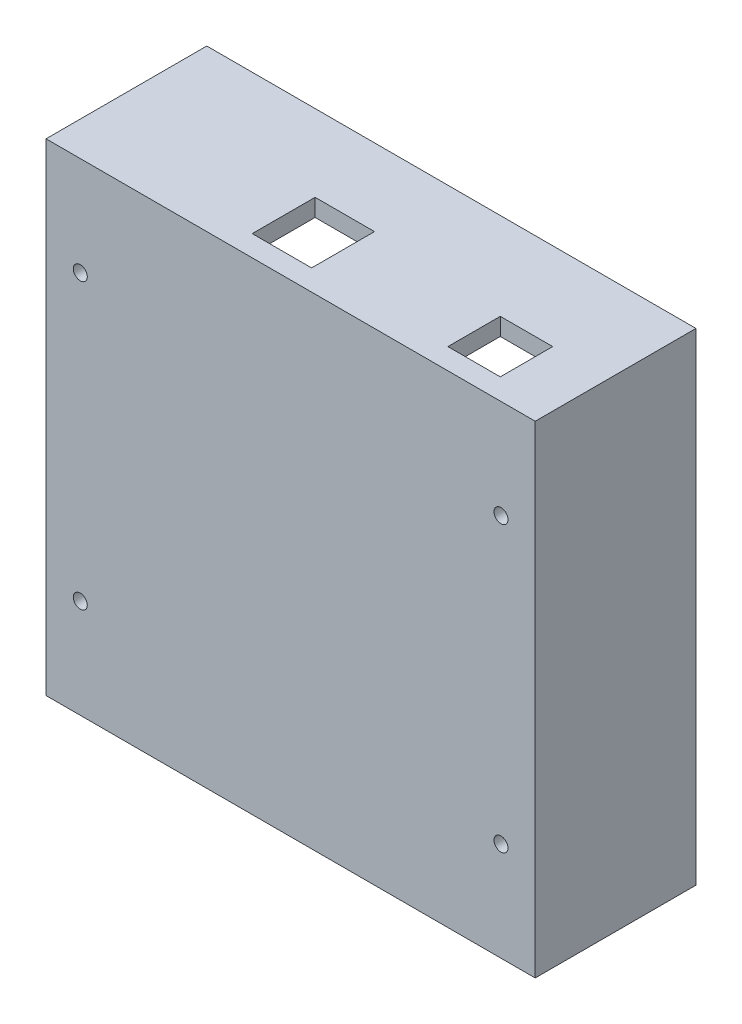
SolidWorks part; units mm, degrees
ref_plane "Front Plane" through (0, 0, 0) normal (0, 0, 1) x (1, 0, 0)
ref_plane "Top Plane" through (0, 0, 0) normal (0, 1, 0) x (1, 0, 0)
ref_plane "Right Plane" through (0, 0, 0) normal (1, 0, 0) x (0, 0, -1)
other "Configuration Table"
sketch "Sketch1" plane through (0, 0, 0) normal (0, 0, 1) x (1, 0, 0)
  line L1 (-47.3118, 118.1115) -> (92.6882, 118.1115)
  line L2 (-47.3118, 118.1115) -> (-47.3118, -19.8885)
  line L3 (-47.3118, -19.8885) -> (92.6882, -19.8885)
  line L4 (92.6882, 118.1115) -> (92.6882, -19.8885)
extrude "Boss-Extrude1" add sketch "Sketch1" along normal blind 46
shell "Shell1" thickness 5
sketch "Sketch8" plane through (0, 118.1115, 0) normal (0, 1, 0) x (1, 0, 0)
  line L0 (-47.3118, -46) -> (-39.3118, -46)
  line L1 (92.6882, -46) -> (-47.3118, -46) construction
sketch "Sketch9" plane through (0, 118.1115, 0) normal (0, 1, 0) x (1, 0, 0)
  line L0 (-39.3118, -46) -> (-39.3118, -40)
  line L6 (-39.3118, -40) -> (-29.3118, -40)
  line L7 (-39.3118, -40) -> (-39.3118, -30)
  line L8 (-39.3118, -30) -> (-29.3118, -30)
  line L9 (-29.3118, -40) -> (-29.3118, -30)
extrude "Cut-Extrude2" cut sketch "Sketch9" against normal blind 5 contours L6 L9 L8 L7
sketch "Sketch10" plane through (0, 118.1115, 0) normal (0, 1, 0) x (1, 0, 0)
  line L0 (-29.3118, -40) -> (-27.3118, -40)
  line L2 (-27.3118, -40) -> (3.6882, -40)
  line L3 (-27.3118, -40) -> (-27.3118, -18)
  line L4 (-27.3118, -18) -> (3.6882, -18)
  line L5 (3.6882, -40) -> (3.6882, -18)
extrude "Cut-Extrude3" cut sketch "Sketch10" against normal blind 5 contours L2 L5 L4 L3
sketch "Sketch11" plane through (0, 118.1115, 0) normal (0, 1, 0) x (1, 0, 0)
  line L0 (3.6882, -40) -> (5.6882, -40)
  line L2 (5.6882, -40) -> (22.6882, -40)
  line L3 (5.6882, -40) -> (5.6882, -22)
  line L4 (5.6882, -22) -> (22.6882, -22)
  line L5 (22.6882, -40) -> (22.6882, -22)
extrude "Cut-Extrude4" cut sketch "Sketch11" against normal blind 5 contours L2 L5 L4 L3
sketch "Sketch12" plane through (0, 118.1115, 0) normal (0, 1, 0) x (1, 0, 0)
  line L0 (22.6882, -40) -> (26.6882, -40)
  line L2 (26.6882, -40) -> (58.6882, -40)
  line L3 (26.6882, -40) -> (26.6882, -27)
  line L4 (26.6882, -27) -> (58.6882, -27)
  line L5 (58.6882, -40) -> (58.6882, -27)
extrude "Cut-Extrude5" cut sketch "Sketch12" against normal blind 5 contours L2 L5 L4 L3
sketch "Sketch13" plane through (0, 118.1115, 0) normal (0, 1, 0) x (1, 0, 0)
  line L0 (58.6882, -40) -> (61.6882, -40)
  line L2 (61.6882, -40) -> (76.6882, -40)
  line L3 (61.6882, -40) -> (61.6882, -25)
  line L4 (61.6882, -25) -> (76.6882, -25)
  line L5 (76.6882, -40) -> (76.6882, -25)
extrude "Cut-Extrude6" cut sketch "Sketch13" against normal blind 5 contours L2 L5 L4 L3
sketch "Sketch19" plane through (0, 0, 46) normal (0, 0, 1) x (1, 0, 0)
  circle A2 centre (-37.5118, 8.4115) radius 2
  circle A4 centre (-37.5118, 89.8115) radius 2
  circle A5 centre (82.8882, 8.4115) radius 2
  circle A6 centre (82.8882, 89.8115) radius 2
extrude "Cut-Extrude8" cut sketch "Sketch19" against normal blind 5
sketch "Sketch21" plane through (0, -19.8885, 0) normal (0, -1, 0) x (1, 0, 0)
  line L2 (-28.3118, 40) -> (-12.3118, 40)
  line L3 (-28.3118, 40) -> (-28.3118, 24)
  line L4 (-28.3118, 24) -> (-12.3118, 24)
  line L5 (-12.3118, 40) -> (-12.3118, 24)
extrude "Cut-Extrude11" cut sketch "Sketch21" against normal blind 5
sketch "Sketch23" plane through (0, -19.8885, 0) normal (0, -1, 0) x (1, 0, 0)
  line L2 (-8.3118, 40) -> (7.6882, 40)
  line L3 (-8.3118, 40) -> (-8.3118, 24)
  line L4 (-8.3118, 24) -> (7.6882, 24)
  line L5 (7.6882, 40) -> (7.6882, 24)
extrude "Cut-Extrude12" cut sketch "Sketch23" against normal blind 5
sketch "Sketch24" plane through (0, 118.1115, 0) normal (0, 1, 0) x (1, 0, 0)
  line L1 (-39.3118, -30) -> (-29.3118, -30)
  line L2 (-39.3118, -30) -> (-39.3118, -40)
  line L3 (-39.3118, -40) -> (-29.3118, -40)
  line L4 (-29.3118, -30) -> (-29.3118, -40)
  line L5 (-27.3118, -18) -> (3.6882, -18)
  line L6 (-27.3118, -18) -> (-27.3118, -40)
  line L7 (-27.3118, -40) -> (3.6882, -40)
  line L8 (3.6882, -18) -> (3.6882, -40)
  line L9 (26.6882, -27) -> (58.6882, -27)
  line L10 (26.6882, -27) -> (26.6882, -40)
  line L11 (26.6882, -40) -> (58.6882, -40)
  line L12 (58.6882, -27) -> (58.6882, -40)
extrude "Boss-Extrude2" add sketch "Sketch24" against normal blind 5
